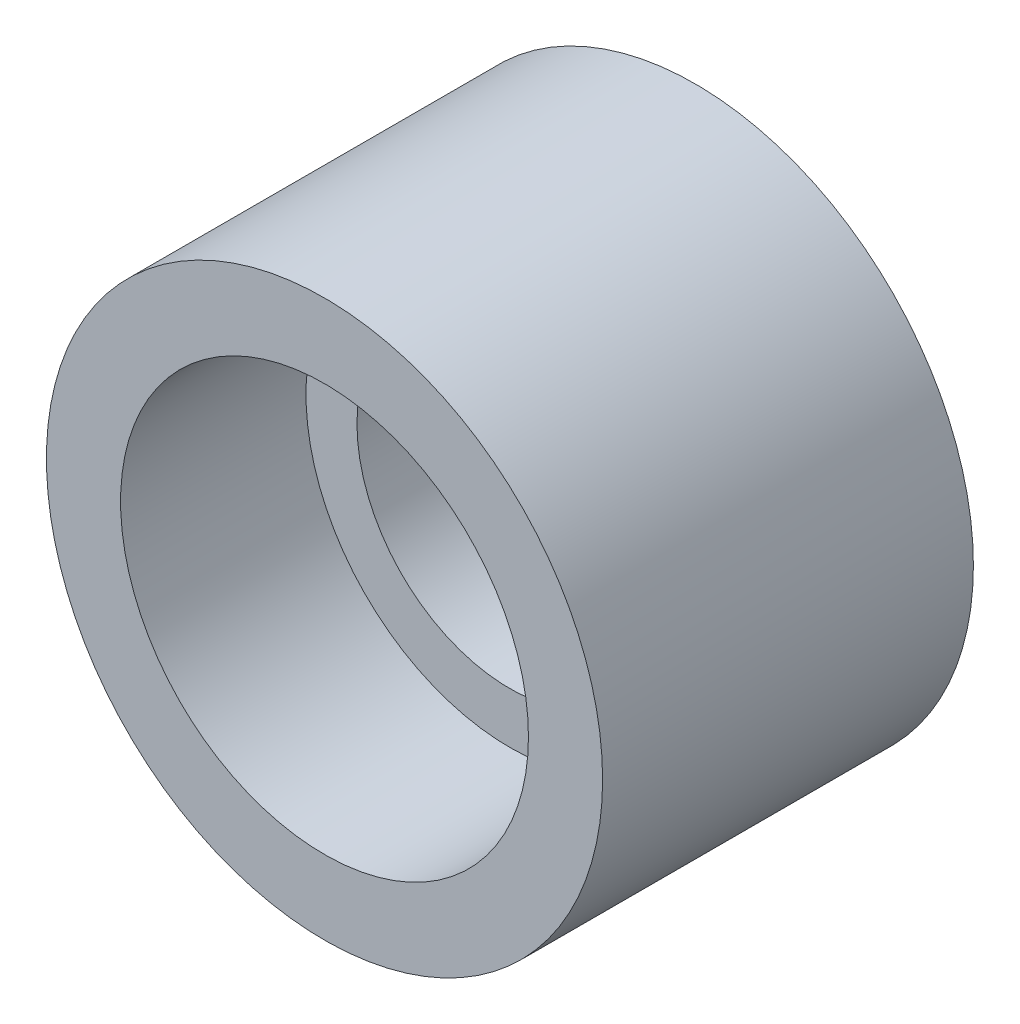
from build123d import *

# Parameters (mm, degrees)
SKETCH1_R                  = 15
BOSS_EXTRUDE1_DEPTH        = 20
SKETCH2_R                  = 11
CUT_EXTRUDE1_DEPTH         = 10
M18X1_5_TAPPED_HOLE1_D     = 16.5
M18X1_5_TAPPED_HOLE1_DEPTH = 40.5
M18X1_5_TAPPED_HOLE1_TIP   = 4.957100107


with BuildPart() as part:
    # Sketch1 → Boss-Extrude1 (new body)
    with BuildSketch(Plane.XY):
        Circle(SKETCH1_R)
    extrude(amount=BOSS_EXTRUDE1_DEPTH)

    # Sketch2 → Cut-Extrude1 (cut)
    with BuildSketch(Plane.XY.offset(20)):
        Circle(SKETCH2_R)
    extrude(amount=-CUT_EXTRUDE1_DEPTH, mode=Mode.SUBTRACT)

    # M18x1.5 Tapped Hole1
    with Locations(Plane(origin=(0, 0, 0), x_dir=(-1, 0, 0), z_dir=(0, 0, -1))):
        with Locations((0, 0)):
            Hole(M18X1_5_TAPPED_HOLE1_D / 2, depth=M18X1_5_TAPPED_HOLE1_DEPTH)
            with Locations((0, 0, -(M18X1_5_TAPPED_HOLE1_DEPTH + M18X1_5_TAPPED_HOLE1_TIP / 2))):  # 118° drill point
                Cone(0, M18X1_5_TAPPED_HOLE1_D / 2, M18X1_5_TAPPED_HOLE1_TIP, mode=Mode.SUBTRACT)


solid = part.part
